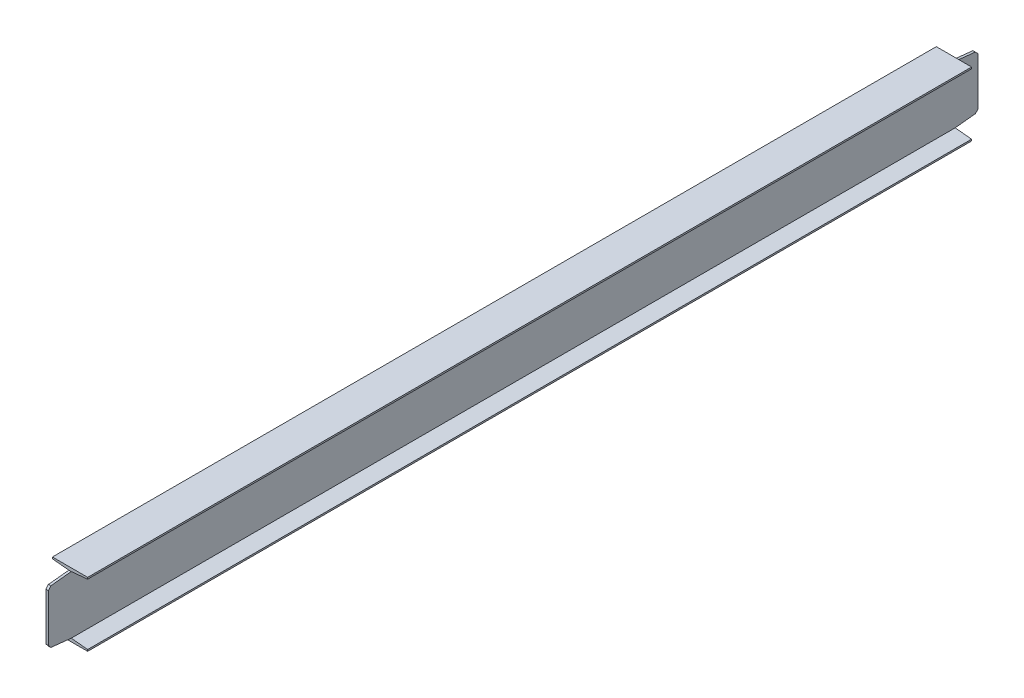
from build123d import *
from OCP.BRepFilletAPI import BRepFilletAPI_MakeChamfer

# Parameters (mm, degrees)
EXTRUDE_1_DEPTH          = 1160
CUT_EXTRUDE_1_DEPTH      = 1164.587555795
CUT_EXTRUDE_1_DEPTH_BACK = 1164.587555795
CHAMFER_1_SIZE           = 6
CHAMFER_1_SIZE2          = 6.742931709


with BuildPart() as part:
    # 草图1 → 凸台-拉伸1 (new, symmetric)
    with BuildSketch(Plane.XY):
        Polygon((44, 80), (-44, 80), (-44, 76), (-3, 72), (-3, -72), (-44, -76), (-44, -80), (44, -80), (44, -76), (3, -72), (3, 72), (44, 76), align=None)
    extrude(amount=EXTRUDE_1_DEPTH, both=True)

    # 草图3 → 切除-拉伸1 (cut, two sides: drawn at the far end of the back side and taken through both)
    with BuildSketch(Plane(origin=(0, 0, 0), x_dir=(0, 0, -1), z_dir=(1, 0, 0)).offset(-CUT_EXTRUDE_1_DEPTH_BACK)):
        Polygon((-1160, 66), (-1103, 72), (-1103, 80), (-1160, 80), align=None)
        Polygon((1160, 80), (1160, 66), (1103, 72), (1103, 80), align=None)
        Polygon((1160, -66), (1103, -72), (1103, -80), (1160, -80), align=None)
        Polygon((-1160, -80), (-1160, -66), (-1103, -72), (-1103, -80), align=None)
    extrude(amount=CUT_EXTRUDE_1_DEPTH + CUT_EXTRUDE_1_DEPTH_BACK, mode=Mode.SUBTRACT)

    # 倒角1: one chamfer whose edges measure the first distance from different faces: ONE call of the kernel's chamfer builder (chamfer() names one face for all edges)
    chamfer_1_edges_1 = [part.edges().sort_by_distance(p)[0] for p in [
        (0, 66, -1160),
        (0, -66, -1160),
    ]]
    chamfer_1_side_1 = [part.faces().sort_by_distance(p)[0] for p in [
        (0, 0, -1160),
    ]]
    chamfer_1_edges_2 = [part.edges().sort_by_distance(p)[0] for p in [
        (0, 66, 1160),
    ]]
    chamfer_1_side_2 = [part.faces().sort_by_distance(p)[0] for p in [
        (0, 69, 1131.5),
    ]]
    chamfer_1_edges_3 = [part.edges().sort_by_distance(p)[0] for p in [
        (0, -66, 1160),
    ]]
    chamfer_1_side_3 = [part.faces().sort_by_distance(p)[0] for p in [
        (0, -69, 1131.5),
    ]]
    chamfer_1 = BRepFilletAPI_MakeChamfer(part.part.solid().wrapped)
    for e in chamfer_1_edges_1:
        chamfer_1.Add(CHAMFER_1_SIZE, CHAMFER_1_SIZE2, e.wrapped, chamfer_1_side_1[0].wrapped)  # the first distance lies on this face
    for e in chamfer_1_edges_2:
        chamfer_1.Add(CHAMFER_1_SIZE, CHAMFER_1_SIZE2, e.wrapped, chamfer_1_side_2[0].wrapped)  # the first distance lies on this face
    for e in chamfer_1_edges_3:
        chamfer_1.Add(CHAMFER_1_SIZE, CHAMFER_1_SIZE2, e.wrapped, chamfer_1_side_3[0].wrapped)  # the first distance lies on this face
    add(Compound.cast(chamfer_1.Shape()), mode=Mode.REPLACE)


solid = part.part
